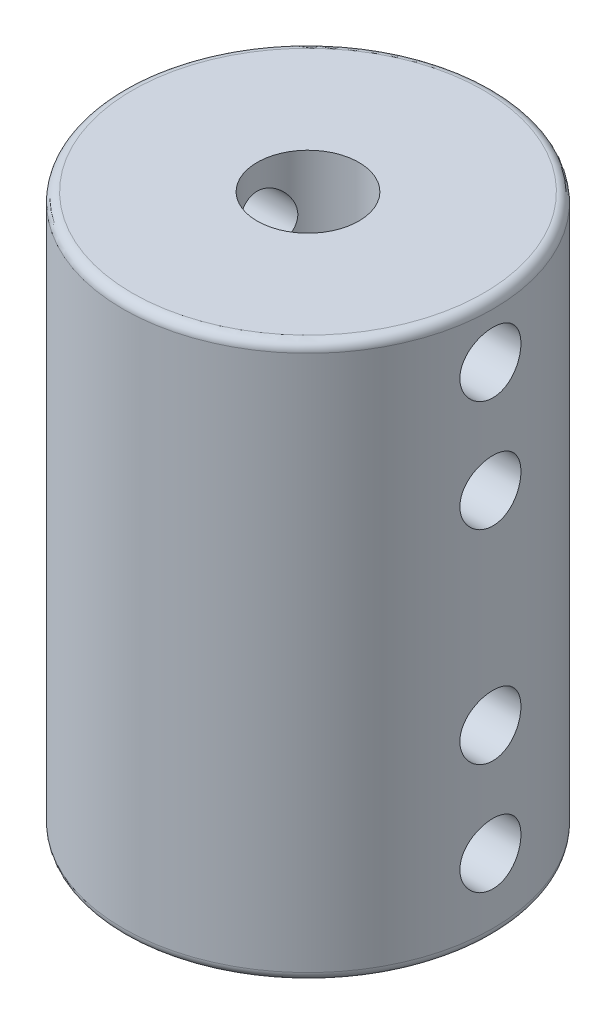
SolidWorks part; units mm, degrees
ref_plane "Front Plane" through (0, 0, 0) normal (0, 0, 1) x (1, 0, 0)
ref_plane "Top Plane" through (0, 0, 0) normal (0, 1, 0) x (1, 0, 0)
ref_plane "Right Plane" through (0, 0, 0) normal (1, 0, 0) x (0, 0, -1)
sketch "Sketch1" plane through (0, 0, 0) normal (0, 1, 0) x (1, 0, 0)
  circle A0 centre (0, 0) radius 10
  dimension "D1" = 20
extrude "Boss-Extrude1" add sketch "Sketch1" along normal blind 30
sketch "Sketch2" plane through (0, 30, 0) normal (0, 1, 0) x (1, 0, 0)
  circle A0 centre (0, 0) radius 2.75
  dimension "D1" = 5.5
extrude "Cut-Extrude1" cut sketch "Sketch2" against normal blind 15
sketch "Sketch3" plane through (0, 0, 0) normal (0, -1, 0) x (1, 0, 0)
  circle A0 centre (0, 0) radius 6
  dimension "D1" = 12
extrude "Cut-Extrude2" cut sketch "Sketch3" against normal blind 15
hole_wizard "M4 Tapped Hole1" positions "3DSketch1" profile "Sketch4" tap size "M4" standard "GB" end condition through all
sketch3d "3DSketch1"
  line L0 (0, 0, 0) -> (10, 0, 0) construction
  circle A1 centre (0, 0, 0) radius 10 construction
  point P0 (10, 4, 0)
  point P2 (10, 10, 0)
  point P4 (10, 27, 0)
  point P6 (10, 21, 0)
  point P19 (0, 10, 0)
  dimension "D1" = 6
  dimension "D2" = 6
  dimension "D3" = 4
  dimension "D4" = 11
cosmetic thread "Hole Thread5" parameters "D2"=4
cosmetic thread "Hole Thread6" parameters "D2"=4
cosmetic thread "Hole Thread7" parameters "D2"=4
cosmetic thread "Hole Thread8" parameters "D2"=4
sketch "Sketch4" plane through (10, 4, 0) normal (0, 1, 0) x (0, 0, -1)
  line L0 (0, 0) -> (0, 20)
  line L1 (0, 20) -> (1.65, 20)
  line L2 (1.65, 20) -> (1.65, 0)
  line L5 (1.65, 0) -> (0, 0)
  line L11 (0, -6.35) -> (0, 107.95) construction
  dimension "通孔螺纹孔钻头直径" = 3.3
  dimension "通孔螺纹孔钻头深度" = 20
fillet "Fillet1" radius 0.5 2 edges at (0, 0, 10) (0, 30, 10)
